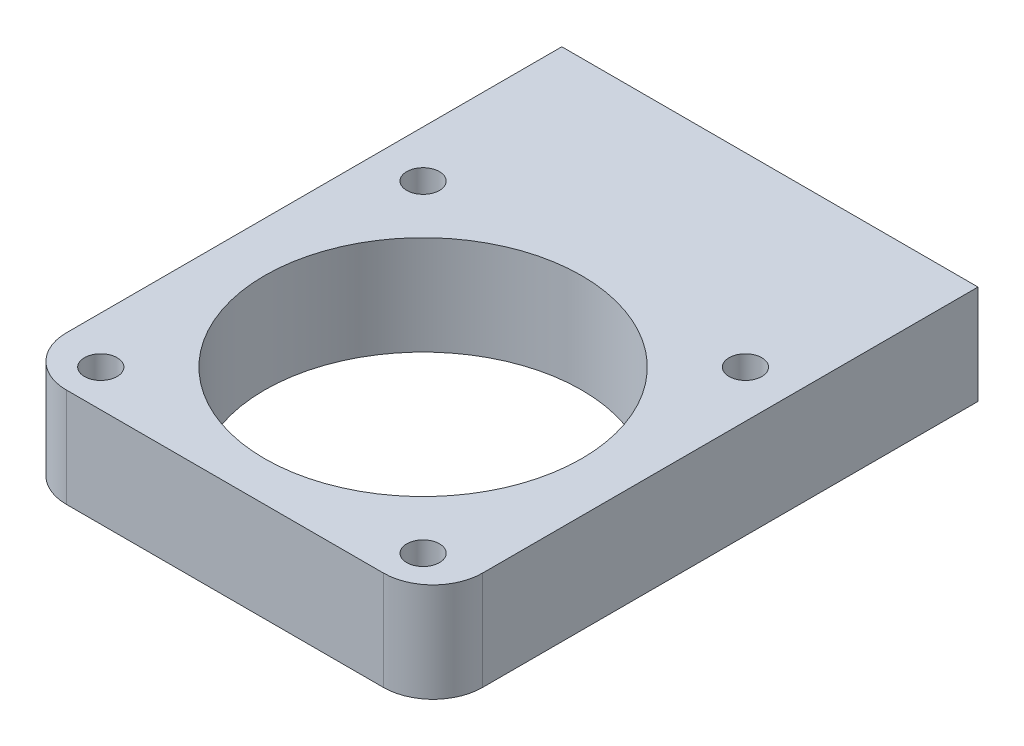
SolidWorks part; units mm, degrees
material "6061铝"
ref_plane "前视基准面" through (0, 0, 0) normal (0, 0, 1) x (1, 0, 0)
ref_plane "上视基准面" through (0, 0, 0) normal (0, 1, 0) x (1, 0, 0)
ref_plane "右视基准面" through (0, 0, 0) normal (1, 0, 0) x (0, 0, -1)
sketch "草图1" plane through (0, 0, 0) normal (0, 1, 0) x (1, 0, 0)
  line L1 (-21, 36) -> (21, 36)
  line L2 (-21, 36) -> (-21, -36)
  line L3 (-21, -36) -> (21, -36)
  line L4 (21, 36) -> (21, -36)
  line L5 (-21, 36) -> (21, -36) construction
  line L6 (-21, -36) -> (21, 36) construction
  point P0 (0, 0)
  dimension "D1" = 42
  dimension "D2" = 72
extrude "凸台-拉伸1" add sketch "草图1" along normal mid plane 10
hole_wizard "M4 螺纹孔2" positions "草图5" profile "草图4" tap size "M4" standard "GB"
sketch "草图5" plane through (0, 0, -36) normal (0, 0, -1) x (-1, 0, 0)
  line L0 (-15, 0) -> (15, 0) construction
  line L1 (-21, 5) -> (-21, -5) construction
  point P0 (-15, 0)
  point P2 (15, 0)
  dimension "D1" = 6
sketch "草图4" plane through (15, 0, -36) normal (1, 0, 0) x (0, 1, 0)
  line L0 (0, 0) -> (0, 12.9914)
  line L1 (0, 12.9914) -> (1.65, 12)
  line L2 (1.65, 12) -> (1.65, 0)
  line L5 (1.65, 0) -> (0, 0)
  line L10 (0, 12.9914) -> (-1.65, 12) construction
  line L11 (0, -6.35) -> (0, 107.95) construction
  dimension "螺纹孔钻头直径" = 3.3
  dimension "螺纹孔钻头深度" = 12
  dimension "导头角度" = 118
cosmetic thread "孔螺蚊线2" parameters "D1"=8, "D2"=4
cosmetic thread "孔螺蚊线3" parameters "D1"=8, "D2"=4
chamfer "倒角1" [suppressed] distance 2 angle 45
sketch "草图6" plane through (0, 5, 0) normal (0, 1, 0) x (1, 0, 0)
  line L1 (21, 36) -> (-21, 36) construction
  circle A0 centre (0, 1) radius 16
  dimension "D1" = 32
  dimension "D2" = 35
extrude "切除-拉伸1" cut sketch "草图6" against normal through all
chamfer "倒角2" distance 10 angle 45 2 edges at (-21, 0, 36) (21, 0, 36)
fillet "圆角1" radius 5 4 edges at (-11, 0, 36) (-21, 0, 26) (11, 0, 36) (21, 0, 26)
sketch "草图15" plane through (0, 5, 0) normal (0, 1, 0) x (1, 0, 0)
  line L0 (21, 36) -> (-21, 36) construction
  line L1 (-32.6097, -19) -> (45.0772, -19)
  line L2 (-32.6097, -19) -> (-32.6097, -71.9081)
  line L3 (-32.6097, -71.9081) -> (45.0772, -71.9081)
  line L4 (45.0772, -19) -> (45.0772, -71.9081)
  dimension "D1" = 55
extrude "切除-拉伸3" cut sketch "草图15" against normal blind 31
fillet "圆角2" radius 5 2 edges at (-21, 0, 19) (21, 0, 19)
hole_wizard "M4 螺纹孔1" positions "草图16" profile "草图17" tap size "M4" standard "GB" end condition through all
sketch "草图16" plane through (0, 5, 0) normal (0, 1, 0) x (1, 0, 0)
  line L0 (0, 1) -> (0, 17) construction
  line L3 (0, 1) -> (16, 1) construction
  circle A0 centre (0, 1) radius 16 construction
  point P0 (-16.265, 17.265)
  point P2 (16.265, 17.265)
  point P4 (-16.265, -15.265)
  point P6 (16.265, -15.265)
  dimension "D1" = 32.53
  dimension "D2" = 32.53
sketch "草图17" plane through (-16.265, 5, -17.265) normal (1, 0, 0) x (0, 0, 1)
  line L0 (0, 0) -> (0, 10)
  line L1 (0, 10) -> (1.65, 10)
  line L2 (1.65, 10) -> (1.65, 0)
  line L5 (1.65, 0) -> (0, 0)
  line L11 (0, -6.35) -> (0, 107.95) construction
  dimension "通孔螺纹孔钻头直径" = 3.3
  dimension "通孔螺纹孔钻头深度" = 10
cosmetic thread "孔螺蚊线4" parameters "D2"=4
cosmetic thread "孔螺蚊线5" parameters "D2"=4
cosmetic thread "孔螺蚊线6" parameters "D2"=4
cosmetic thread "孔螺蚊线7" parameters "D2"=4
